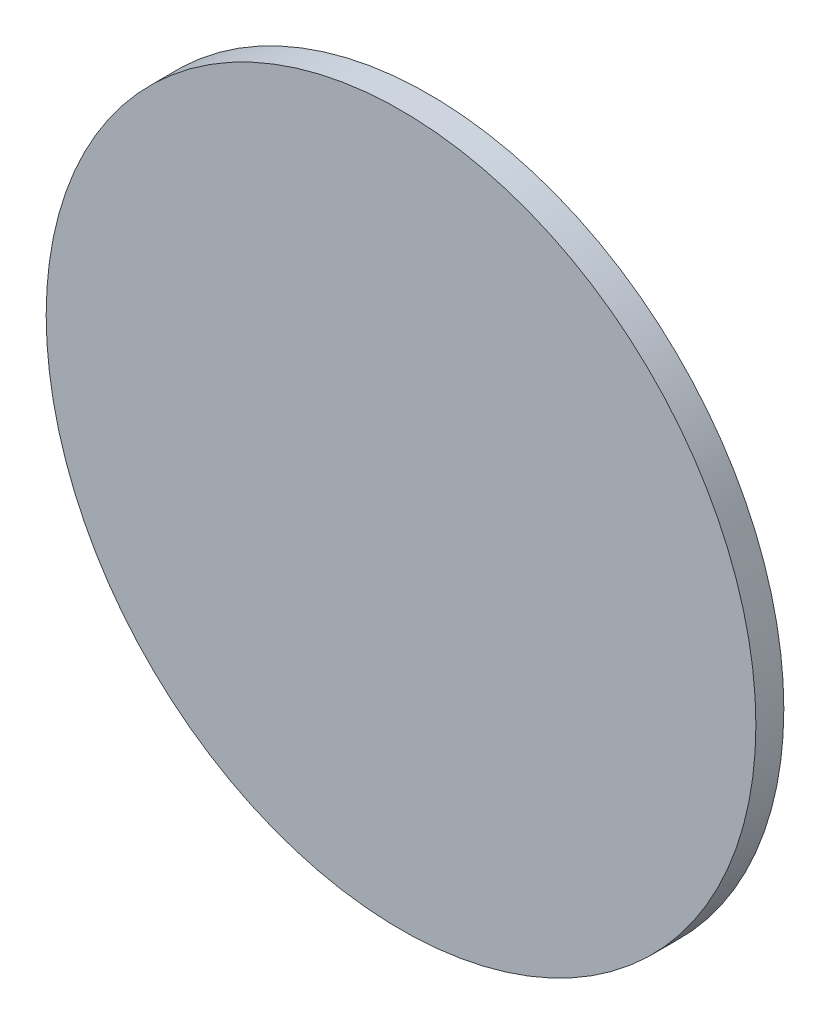
from build123d import *

# Parameters (mm, degrees)
SKETCH1_R           = 12.7
BOSS_EXTRUDE1_DEPTH = 1


with BuildPart() as part:
    # Sketch1 → Boss-Extrude1 (new body)
    with BuildSketch(Plane.XY):
        with Locations((28.2, -28.2)):
            Circle(SKETCH1_R)
    extrude(amount=BOSS_EXTRUDE1_DEPTH)


solid = part.part
